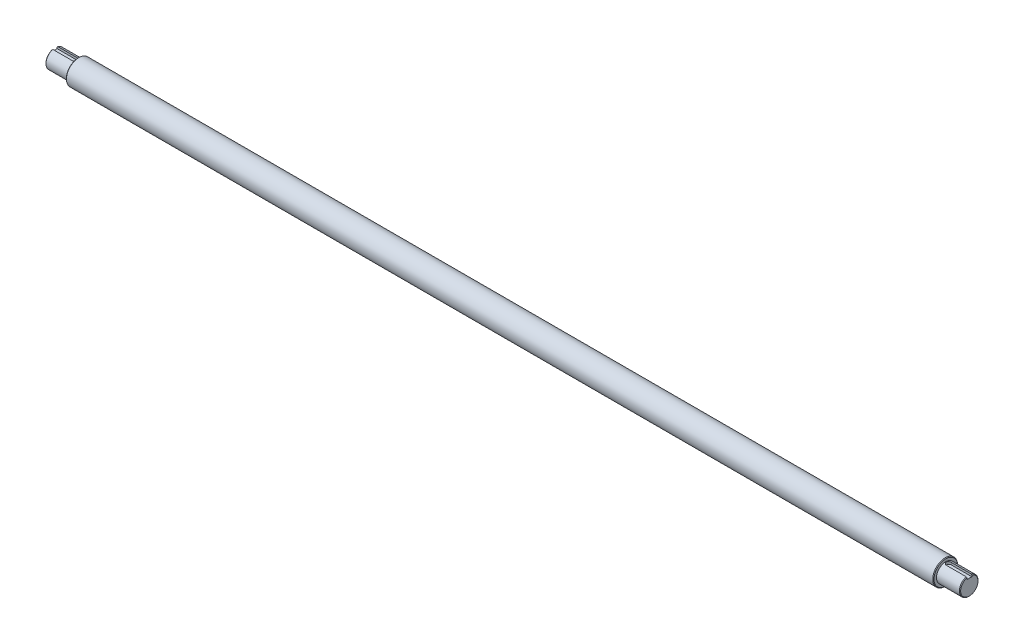
SolidWorks part; units mm, degrees
material "45#"
ref_plane "Front" through (0, 0, 0) normal (0, 0, 1) x (1, 0, 0)
ref_plane "Top" through (0, 0, 0) normal (0, 1, 0) x (1, 0, 0)
ref_plane "Right" through (0, 0, 0) normal (1, 0, 0) x (0, 0, -1)
sketch "Sketch1" plane through (0, 0, 0) normal (0, 0, 1) x (1, 0, 0)
  line L0 (-738, 15) -> (-700, 15)
  line L1 (-700, 15) -> (-700, 20)
  line L2 (-700, 20) -> (700, 20)
  line L3 (700, 20) -> (700, 15)
  line L4 (700, 15) -> (738, 15)
  line L5 (-151.0352, 0) -> (288.7935, 0) construction
  line L6 (738, 15) -> (738, 0)
  line L7 (738, 0) -> (-738, 0)
  line L8 (-738, 0) -> (-738, 15)
  line L9 (0, 0) -> (0, 55.3153) construction
  dimension "D1" = 38
  dimension "D2" = 1400
  dimension "D3" = 20
  dimension "D4" = 15
  dimension "D5" = 38
  dimension "D6" = 15
revolve "Revolve1" add sketch "Sketch1" angle 360 about L7
ref_plane "Plane1" through (0, 0, 0) normal (-1, 0, 0) x (0, 0, 1)
sketch "Sketch2" plane through (-738, 0, 0) normal (-1, 0, 0) x (0, 0, 1)
  line L0 (0, 15) -> (0, 0)
  circle A0 centre (0, 0) radius 15 construction
ref_plane "Plane2" through (0, 15, 0) normal (0, 1, 0) x (1, 0, 0)
sketch "Sketch3" plane through (0, 15, 0) normal (0, 1, 0) x (1, 0, 0)
  line L0 (-738, 0) -> (-92.6704, 0) construction
  line L1 (-738, 15) -> (-738, -15) construction
  line L2 (-700, 15) -> (-700, -15) construction
  line L3 (-705, 4) -> (-738, 4)
  line L4 (-738, 4) -> (-738, -4)
  line L5 (-738, -4) -> (-705, -4)
  arc A1 (-705, -4) -> (-705, 4) centre (-705, 0) ccw
  dimension "D1" = 8
  dimension "D2" = 5
extrude "Cut-Extrude1" cut sketch "Sketch3" against normal blind 4
mirror "Mirror1" about plane through (0, 0, 0) normal (-1, 0, 0) of "Cut-Extrude1"
chamfer "Chamfer1" distance 1 angle 45 4 edges at (-700, 0, -20) (-738, -15, 0) (738, -15, 0) (700, 0, -20)
equation "\"零件重量\"= IIF ( \"SW-质量\" > 100 , int ( \"SW-质量\" ) , \"SW-质量\" )"
